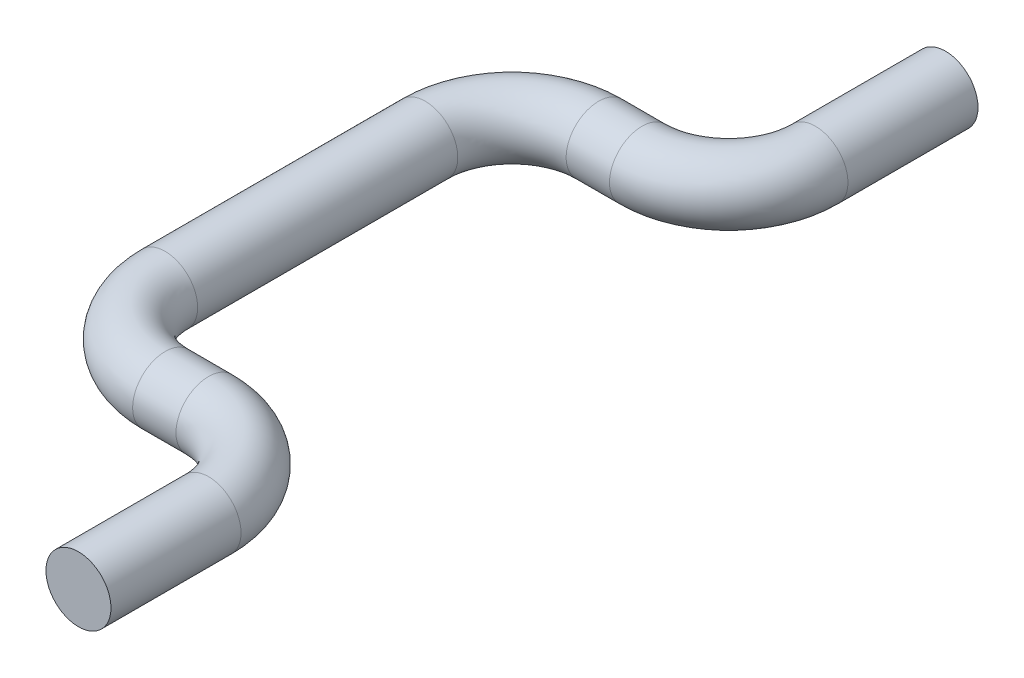
from build123d import *

# Parameters (mm, degrees)
SKETCH2_R = 6


with BuildPart() as part:
    # Sweep1: sweep along a path in Sketch1
    with BuildLine(Plane(origin=(0, 0, 0), x_dir=(1, 0, 0), z_dir=(0, 1, 0))) as sweep1_path:
        Line((0, 160), (0, 136))
        ThreePointArc((0, 136), (-4.686291501, 124.686291501), (-16, 120))
        Line((-16, 120), (-24, 120))
        ThreePointArc((-24, 120), (-35.313708499, 115.313708499), (-40, 104))
        Line((-40, 104), (-40, 56))
        ThreePointArc((-40, 56), (-35.313708499, 44.686291501), (-24, 40))
        Line((-24, 40), (-16, 40))
        ThreePointArc((-16, 40), (-4.686291501, 35.313708499), (0, 24))
        Line((0, 24), (0, 0))
    # Sketch2 → Sweep1 (sweep)
    with BuildSketch(Plane.XY):
        Circle(SKETCH2_R)
    sweep(path=sweep1_path.line)


solid = part.part
